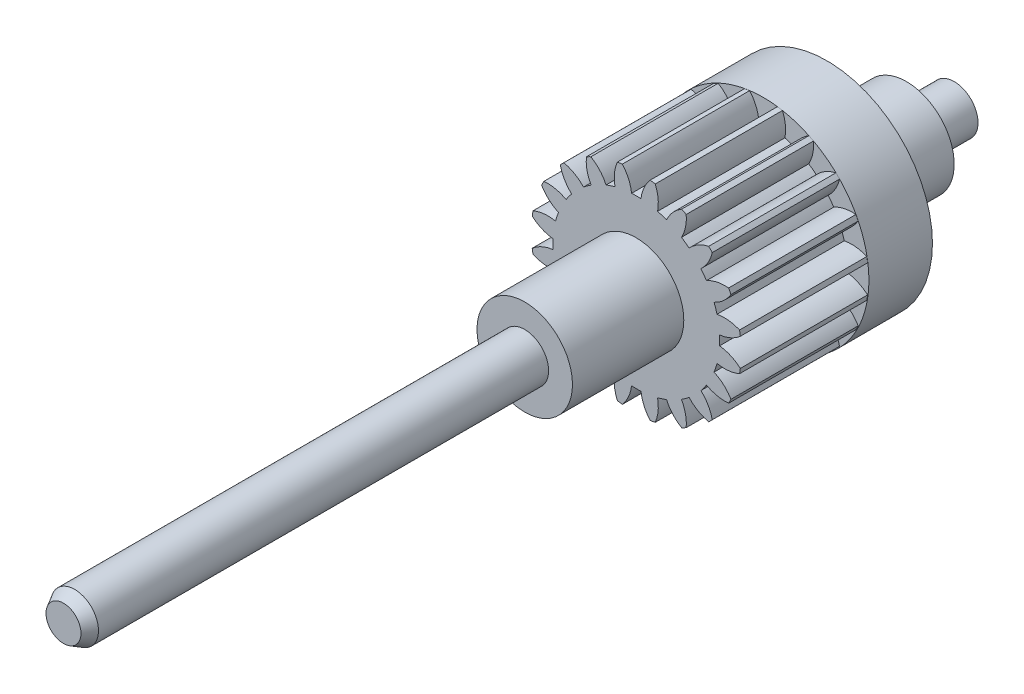
SolidWorks part; units mm, degrees
ref_plane "Front plane" through (0, 0, 0) normal (0, 0, 1) x (1, 0, 0)
ref_plane "Top plane" through (0, 0, 0) normal (0, 1, 0) x (1, 0, 0)
ref_plane "Right plane" through (0, 0, 0) normal (1, 0, 0) x (0, 0, -1)
sketch "Sketch 1" plane through (0, 0, 0) normal (0, 0, 1) x (1, 0, 0)
  arc A492 (-3.2649, 0.453) -> (-2.6138, 0.164) centre (-2.4744, 1.3559) ccw
  arc A493 (-2.6138, 0.164) -> (-2.6138, -0.1315) centre (0.0061, 0.0162) ccw
  arc A494 (-2.6138, -0.1315) -> (-3.2649, -0.4206) centre (-2.4744, -1.3234) ccw
  arc A495 (-3.2649, -0.4206) -> (-3.2398, -0.5791) centre (0.0061, 0.0162) ccw
  arc A496 (-3.2398, -0.5791) -> (-2.5312, -0.6528) centre (-2.7669, 0.5238) ccw
  arc A497 (-2.5312, -0.6528) -> (-2.4399, -0.9339) centre (0.0061, 0.0162) ccw
  arc A498 (-2.4399, -0.9339) -> (-2.9698, -1.41) centre (-1.939, -2.0243) ccw
  arc A499 (-2.9698, -1.41) -> (-2.8969, -1.553) centre (0.0061, 0.0162) ccw
  arc A500 (-2.8969, -1.553) -> (-2.2003, -1.4041) centre (-2.7881, -0.358) ccw
  arc A501 (-2.2003, -1.4041) -> (-2.0266, -1.6432) centre (0.0061, 0.0162) ccw
  arc A502 (-2.0266, -1.6432) -> (-2.3834, -2.2598) centre (-1.2132, -2.5255) ccw
  arc A503 (-2.3834, -2.2598) -> (-2.2699, -2.3733) centre (0.0061, 0.0162) ccw
  arc A504 (-2.2699, -2.3733) -> (-1.6534, -2.0164) centre (-2.5357, -1.2031) ccw
  arc A505 (-1.6534, -2.0164) -> (-1.4143, -2.1901) centre (0.0061, 0.0162) ccw
  arc A506 (-1.4143, -2.1901) -> (-1.5632, -2.8868) centre (-0.3681, -2.7779) ccw
  arc A507 (-1.5632, -2.8868) -> (-1.4201, -2.9597) centre (0.0061, 0.0162) ccw
  arc A508 (-1.4201, -2.9597) -> (-0.944, -2.4297) centre (-2.0345, -1.9288) ccw
  arc A509 (-0.944, -2.4297) -> (-0.663, -2.521) centre (0.0061, 0.0162) ccw
  arc A510 (-0.663, -2.521) -> (-0.5893, -3.2296) centre (0.5136, -2.7568) ccw
  arc A511 (-0.5893, -3.2296) -> (-0.4307, -3.2547) centre (0.0061, 0.0162) ccw
  arc A512 (-0.4307, -3.2547) -> (-0.1417, -2.6036) centre (-1.3335, -2.4642) ccw
  arc A513 (-0.1417, -2.6036) -> (0.1538, -2.6036) centre (0.0061, 0.0162) ccw
  arc A514 (0.1538, -2.6036) -> (0.4429, -3.2547) centre (1.3457, -2.4642) ccw
  arc A515 (0.4429, -3.2547) -> (0.6014, -3.2296) centre (0.0061, 0.0162) ccw
  arc A516 (0.6014, -3.2296) -> (0.6751, -2.521) centre (-0.5015, -2.7568) ccw
  arc A517 (0.6751, -2.521) -> (0.9562, -2.4297) centre (0.0061, 0.0162) ccw
  arc A518 (0.9562, -2.4297) -> (1.4323, -2.9597) centre (2.0466, -1.9288) ccw
  arc A519 (1.4323, -2.9597) -> (1.5753, -2.8868) centre (0.0061, 0.0162) ccw
  arc A520 (1.5753, -2.8868) -> (1.4264, -2.1901) centre (0.3803, -2.7779) ccw
  arc A521 (1.4264, -2.1901) -> (1.6655, -2.0164) centre (0.0061, 0.0162) ccw
  arc A522 (1.6655, -2.0164) -> (2.2821, -2.3733) centre (2.5478, -1.2031) ccw
  arc A523 (2.2821, -2.3733) -> (2.3956, -2.2598) centre (0.0061, 0.0162) ccw
  arc A524 (2.3956, -2.2598) -> (2.0387, -1.6432) centre (1.2254, -2.5255) ccw
  arc A525 (2.0387, -1.6432) -> (2.2124, -1.4041) centre (0.0061, 0.0162) ccw
  arc A526 (2.2124, -1.4041) -> (2.9091, -1.553) centre (2.8002, -0.358) ccw
  arc A527 (2.9091, -1.553) -> (2.982, -1.41) centre (0.0061, 0.0162) ccw
  arc A528 (2.982, -1.41) -> (2.452, -0.9339) centre (1.9512, -2.0243) ccw
  arc A529 (2.452, -0.9339) -> (2.5433, -0.6528) centre (0.0061, 0.0162) ccw
  arc A530 (2.5433, -0.6528) -> (3.2519, -0.5791) centre (2.7791, 0.5238) ccw
  arc A531 (3.2519, -0.5791) -> (3.277, -0.4206) centre (0.0061, 0.0162) ccw
  arc A532 (3.277, -0.4206) -> (2.6259, -0.1315) centre (2.4865, -1.3234) ccw
  arc A533 (2.6259, -0.1315) -> (2.6259, 0.164) centre (0.0061, 0.0162) ccw
  arc A534 (2.6259, 0.164) -> (3.277, 0.453) centre (2.4865, 1.3559) ccw
  arc A535 (3.277, 0.453) -> (3.2519, 0.6116) centre (0.0061, 0.0162) ccw
  arc A536 (3.2519, 0.6116) -> (2.5433, 0.6853) centre (2.7791, -0.4913) ccw
  arc A537 (2.5433, 0.6853) -> (2.452, 0.9663) centre (0.0061, 0.0162) ccw
  arc A538 (2.452, 0.9663) -> (2.982, 1.4424) centre (1.9512, 2.0568) ccw
  arc A539 (2.982, 1.4424) -> (2.9091, 1.5855) centre (0.0061, 0.0162) ccw
  arc A540 (2.9091, 1.5855) -> (2.2124, 1.4366) centre (2.8002, 0.3904) ccw
  arc A541 (2.2124, 1.4366) -> (2.0387, 1.6757) centre (0.0061, 0.0162) ccw
  arc A542 (2.0387, 1.6757) -> (2.3956, 2.2922) centre (1.2254, 2.558) ccw
  arc A543 (2.3956, 2.2922) -> (2.2821, 2.4057) centre (0.0061, 0.0162) ccw
  arc A544 (2.2821, 2.4057) -> (1.6655, 2.0489) centre (2.5478, 1.2355) ccw
  arc A545 (1.6655, 2.0489) -> (1.4264, 2.2226) centre (0.0061, 0.0162) ccw
  arc A546 (1.4264, 2.2226) -> (1.5753, 2.9192) centre (0.3803, 2.8104) ccw
  arc A547 (1.5753, 2.9192) -> (1.4323, 2.9921) centre (0.0061, 0.0162) ccw
  arc A548 (1.4323, 2.9921) -> (0.9562, 2.4622) centre (2.0466, 1.9613) ccw
  arc A549 (0.9562, 2.4622) -> (0.6751, 2.5535) centre (0.0061, 0.0162) ccw
  arc A550 (0.6751, 2.5535) -> (0.6014, 3.2621) centre (-0.5015, 2.7892) ccw
  arc A551 (0.6014, 3.2621) -> (0.4429, 3.2872) centre (0.0061, 0.0162) ccw
  arc A552 (0.4429, 3.2872) -> (0.1538, 2.6361) centre (1.3457, 2.4967) ccw
  arc A553 (0.1538, 2.6361) -> (-0.1417, 2.6361) centre (0.0061, 0.0162) ccw
  arc A554 (-0.1417, 2.6361) -> (-0.4307, 3.2872) centre (-1.3335, 2.4967) ccw
  arc A555 (-0.4307, 3.2872) -> (-0.5893, 3.2621) centre (0.0061, 0.0162) ccw
  arc A556 (-0.5893, 3.2621) -> (-0.663, 2.5535) centre (0.5136, 2.7892) ccw
  arc A557 (-0.663, 2.5535) -> (-0.944, 2.4622) centre (0.0061, 0.0162) ccw
  arc A558 (-0.944, 2.4622) -> (-1.4201, 2.9921) centre (-2.0345, 1.9613) ccw
  arc A559 (-1.4201, 2.9921) -> (-1.5632, 2.9192) centre (0.0061, 0.0162) ccw
  arc A560 (-1.5632, 2.9192) -> (-1.4143, 2.2226) centre (-0.3681, 2.8104) ccw
  arc A561 (-1.4143, 2.2226) -> (-1.6534, 2.0489) centre (0.0061, 0.0162) ccw
  arc A562 (-1.6534, 2.0489) -> (-2.2699, 2.4057) centre (-2.5357, 1.2355) ccw
  arc A563 (-2.2699, 2.4057) -> (-2.3834, 2.2922) centre (0.0061, 0.0162) ccw
  arc A564 (-2.3834, 2.2922) -> (-2.0266, 1.6757) centre (-1.2132, 2.558) ccw
  arc A565 (-2.0266, 1.6757) -> (-2.2003, 1.4366) centre (0.0061, 0.0162) ccw
  arc A566 (-2.2003, 1.4366) -> (-2.8969, 1.5855) centre (-2.7881, 0.3904) ccw
  arc A567 (-2.8969, 1.5855) -> (-2.9698, 1.4424) centre (0.0061, 0.0162) ccw
  arc A568 (-2.9698, 1.4424) -> (-2.4399, 0.9663) centre (-1.939, 2.0568) ccw
  arc A569 (-2.4399, 0.9663) -> (-2.5312, 0.6853) centre (0.0061, 0.0162) ccw
  arc A570 (-2.5312, 0.6853) -> (-3.2398, 0.6116) centre (-2.7669, -0.4913) ccw
  arc A571 (-3.2398, 0.6116) -> (-3.2649, 0.453) centre (0.0061, 0.0162) ccw
extrude "Boss-Extrude 1" add sketch "Sketch 1" along normal blind 4
sketch "Sketch 3" plane through (0, 0, 0) normal (0, 0, 1) x (1, 0, 0)
  circle A1 centre (0, 0) radius 3.3172
extrude "Boss-Extrude 2" add sketch "Sketch 3" against normal blind 2
sketch "Sketch 4" plane through (0, 0, -2) normal (0, 0, -1) x (-1, 0, 0)
  circle A0 centre (0, 0) radius 1.5
  circle A1 centre (0, 0) radius 3.3172
  circle A2 centre (0, 0) radius 3.3172
  dimension "D2" = 3
  dimension "D1" = 0
extrude "Boss-Extrude 3" add sketch "Sketch 4" along normal blind 2.5 contours A0
sketch "Sketch 5" plane through (0, 0, 4) normal (0, 0, 1) x (1, 0, 0)
  circle A0 centre (0, 0) radius 1.5
  dimension "D1" = 3
extrude "Boss-Extrude 4" add sketch "Sketch 5" along normal blind 3.5
sketch "Sketch 6" plane through (0, 0, -4.5) normal (0, 0, -1) x (-1, 0, 0)
  circle A0 centre (0, 0) radius 0.75
  dimension "D1" = 1.5
extrude "Boss-Extrude 5" add sketch "Sketch 6" along normal blind 1.5
sketch "Sketch 7" plane through (0, 0, 7.5) normal (0, 0, 1) x (1, 0, 0)
  circle A0 centre (0, 0) radius 0.75
  dimension "D1" = 1.5
extrude "Boss-Extrude 6" add sketch "Sketch 7" along normal blind 14.5
ref_axis "Axis 1" through (0, 0, 22) along (0, 0, -1)
sketch "Sketch 9" plane through (0, 0, 0) normal (0, 1, 0) x (1, 0, 0)
  line L0 (-0.75, -22) -> (0.75, -22) construction
  line L1 (0.55, -22) -> (0.75, -22)
  line L2 (0.55, -22) -> (0.75, -21.65)
  line L3 (0.75, -22) -> (0.75, -7.5) construction
  line L4 (0.75, -22) -> (0.75, -21.65)
  dimension "D1" = 0.2
  dimension "D3" = 0.35
revolve "Cut-Revolve 1" cut sketch "Sketch 9" angle 360 about axis through (0, 0, 22) along (0, 0, -1)
